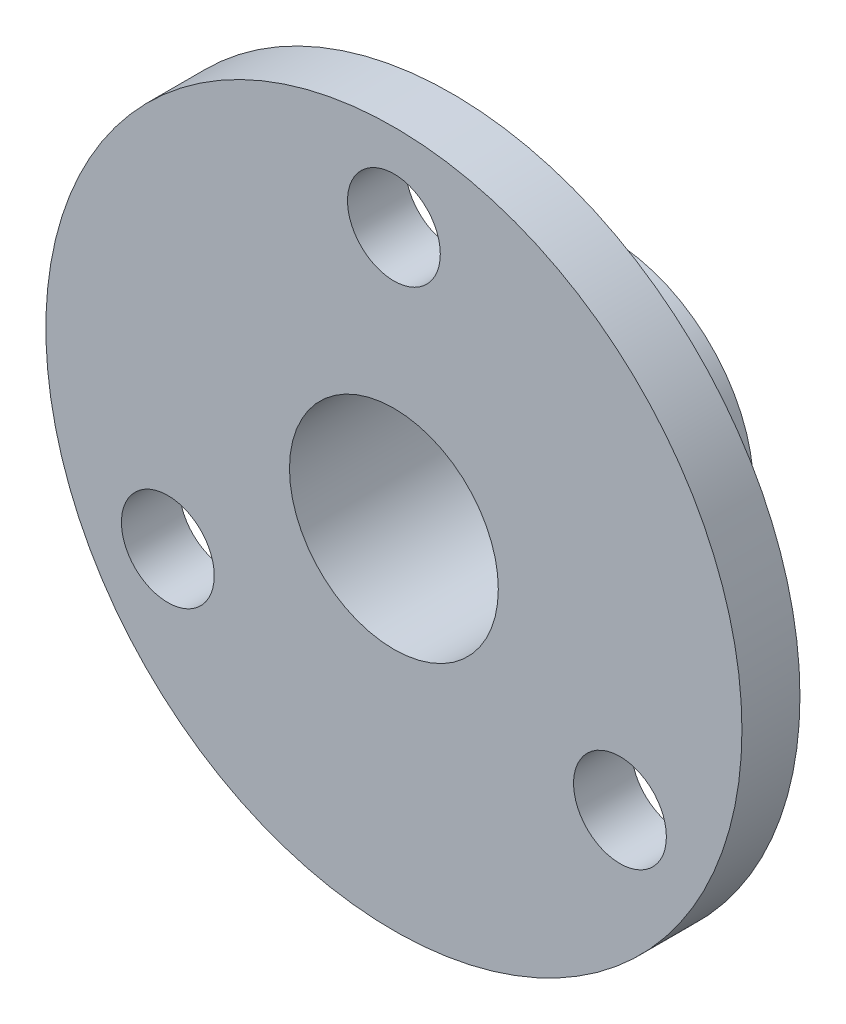
SolidWorks part; units mm, degrees
ref_plane "前视基准面" through (0, 0, 0) normal (0, 0, 1) x (1, 0, 0)
ref_plane "上视基准面" through (0, 0, 0) normal (0, 1, 0) x (1, 0, 0)
ref_plane "右视基准面" through (0, 0, 0) normal (1, 0, 0) x (0, 0, -1)
sketch "草图1" plane through (0, 0, 0) normal (0, 0, 1) x (1, 0, 0)
  circle A0 centre (0, 0) radius 22.5 construction
  circle A1 centre (0, 0) radius 9
  circle A2 centre (0, 0) radius 30
  circle A3 centre (0, 22.5) radius 4
  circle A4 centre (19.4856, -11.25) radius 4
  circle A5 centre (-19.4856, -11.25) radius 4
  point P13 (0, 0)
  dimension "D1" = 45
  dimension "D2" = 18
  dimension "D3" = 60
  dimension "D4" = 8
  dimension "D6" = 33.75
  dimension "D5" = 3
extrude "凸台-拉伸1" add sketch "草图1" along normal blind 5
sketch "草图2" plane through (0, 0, 0) normal (0, 0, -1) x (-1, 0, 0)
  circle A0 centre (0, 0) radius 14
  circle A1 centre (0, 0) radius 9
  dimension "D1" = 28
  dimension "D2" = 18
extrude "凸台-拉伸2" add sketch "草图2" along normal blind 10
sketch "草图3" plane through (0, 0, -10) normal (0, 0, -1) x (-1, 0, 0)
  circle A0 centre (0, 0) radius 12.5
  circle A1 centre (0, 0) radius 8.1
  dimension "D1" = 16.2
  dimension "D2" = 25
extrude "凸台-拉伸3" add sketch "草图3" along normal blind 3.5
